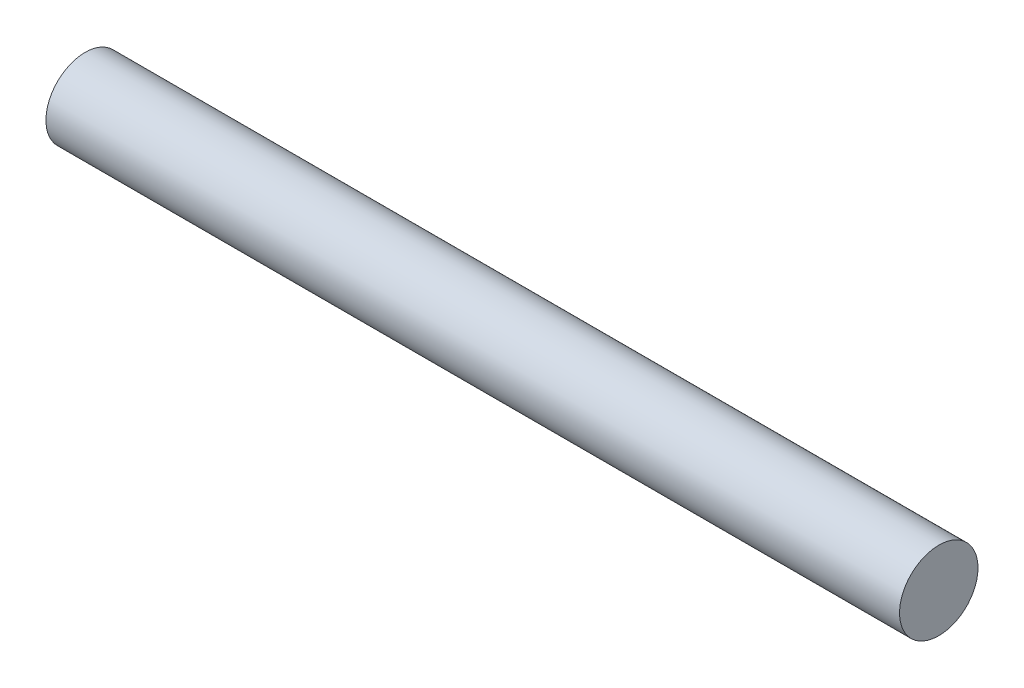
from build123d import *

# Parameters (mm, degrees)
SKETCH_1_R      = 12.5
EXTRUDE_1_DEPTH = 136


with BuildPart() as part:
    # 草图1 → 凸台-拉伸1 (new, symmetric)
    with BuildSketch(Plane(origin=(0, 0, 0), x_dir=(0, 0, -1), z_dir=(1, 0, 0))):
        Circle(SKETCH_1_R)
    extrude(amount=EXTRUDE_1_DEPTH, both=True)


solid = part.part
